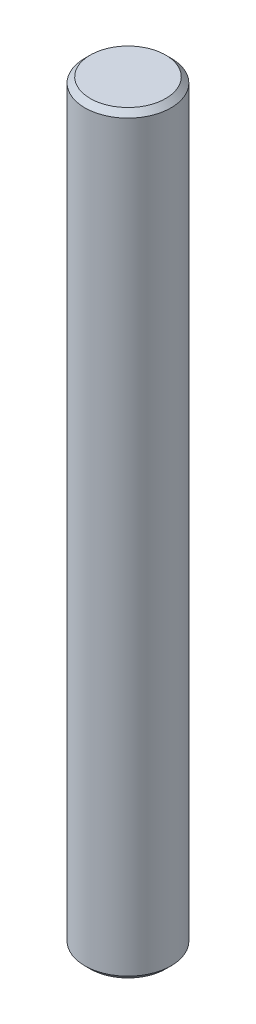
SolidWorks part; units mm, degrees
ref_plane "Front" through (0, 0, 0) normal (0, 0, 1) x (1, 0, 0)
ref_plane "Top" through (0, 0, 0) normal (0, 1, 0) x (1, 0, 0)
ref_plane "Right" through (0, 0, 0) normal (1, 0, 0) x (0, 0, -1)
sketch "草图1" plane through (0, 0, 0) normal (0, 1, 0) x (1, 0, 0)
  circle A0 centre (0, 0) radius 4
  dimension "D1" = 8
extrude "凸台-拉伸1" add sketch "草图1" along normal blind 70
cosmetic thread "装饰螺纹线1" parameters "D1"=15, "D2"=6.647
cosmetic thread "装饰螺纹线2" parameters "D1"=20, "D2"=6.647
chamfer "倒角1" distance 0.5 angle 45 2 edges at (0, 70, 4) (0, 0, 4)
hole_wizard "M4 螺纹孔1" positions "草图3" profile "草图2" tap size "M4" standard "Iso"
sketch "草图3" plane through (0, 0, 0) normal (0, -1, 0) x (-1, 0, 0)
  point P0 (0, 0)
sketch "草图2" plane through (0, 0, 0) normal (1, 0, 0) x (0, 0, -1)
  line L0 (0, 0) -> (0, 15.0914)
  line L1 (0, 15.0914) -> (1.65, 14.1)
  line L2 (1.65, 14.1) -> (1.65, 0)
  line L5 (1.65, 0) -> (0, 0)
  line L10 (0, 15.0914) -> (-1.65, 14.1) construction
  line L11 (0, -6.35) -> (0, 107.95) construction
  dimension "螺纹孔钻头直径" = 3.3
  dimension "螺纹孔钻头深度" = 14.1
  dimension "导头角度" = 118
cosmetic thread "孔螺蚊线1" parameters "D1"=12, "D2"=4
